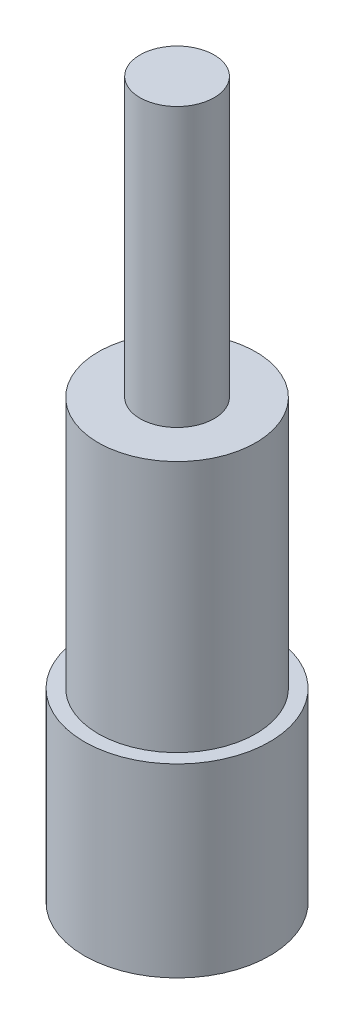
SolidWorks part; units mm, degrees
material "6061-T6 (GB)"
ref_plane "Front Plane" through (0, 0, 0) normal (0, 0, 1) x (1, 0, 0)
ref_plane "Top Plane" through (0, 0, 0) normal (0, 1, 0) x (1, 0, 0)
ref_plane "Right Plane" through (0, 0, 0) normal (1, 0, 0) x (0, 0, -1)
sketch "Sketch1" plane through (0, 0, 0) normal (0, 1, 0) x (1, 0, 0)
  circle A0 centre (0, 0) radius 10
  dimension "D1" = 20
extrude "Boss-Extrude1" add sketch "Sketch1" along normal blind 20
sketch "Sketch2" plane through (0, 20, 0) normal (0, 1, 0) x (1, 0, 0)
  circle A0 centre (0, 0) radius 8.5
  dimension "D1" = 17
extrude "Boss-Extrude2" add sketch "Sketch2" along normal blind 27.2
sketch "Sketch3" plane through (0, 47.2, 0) normal (0, 1, 0) x (1, 0, 0)
  circle A0 centre (0, 0) radius 4
  dimension "D1" = 8
extrude "Boss-Extrude3" add sketch "Sketch3" along normal blind 30
cosmetic thread "Cosmetic Thread1"
ref_plane "Plane1" through (0, 0, -4) normal (0, 0, -1) x (-1, 0, 0)
sketch "Sketch4" plane through (0, 0, -4) normal (0, 0, -1) x (-1, 0, 0)
  line L0 (0, 50.2) -> (0, 64.2) construction
  line L1 (-1, 50.2) -> (-1, 64.2)
  line L2 (1, 50.2) -> (1, 64.2)
  line L3 (8.5, 47.2) -> (-8.5, 47.2) construction
  arc A0 (-1, 50.2) -> (1, 50.2) centre (0, 50.2) ccw
  arc A1 (1, 64.2) -> (-1, 64.2) centre (0, 64.2) ccw
  point P3 (0, 57.2)
  dimension "D2" = 3
  dimension "D1" = 2
  dimension "D3" = 14
extrude "Cut-Extrude1" cut sketch "Sketch4" against normal blind 1.2
